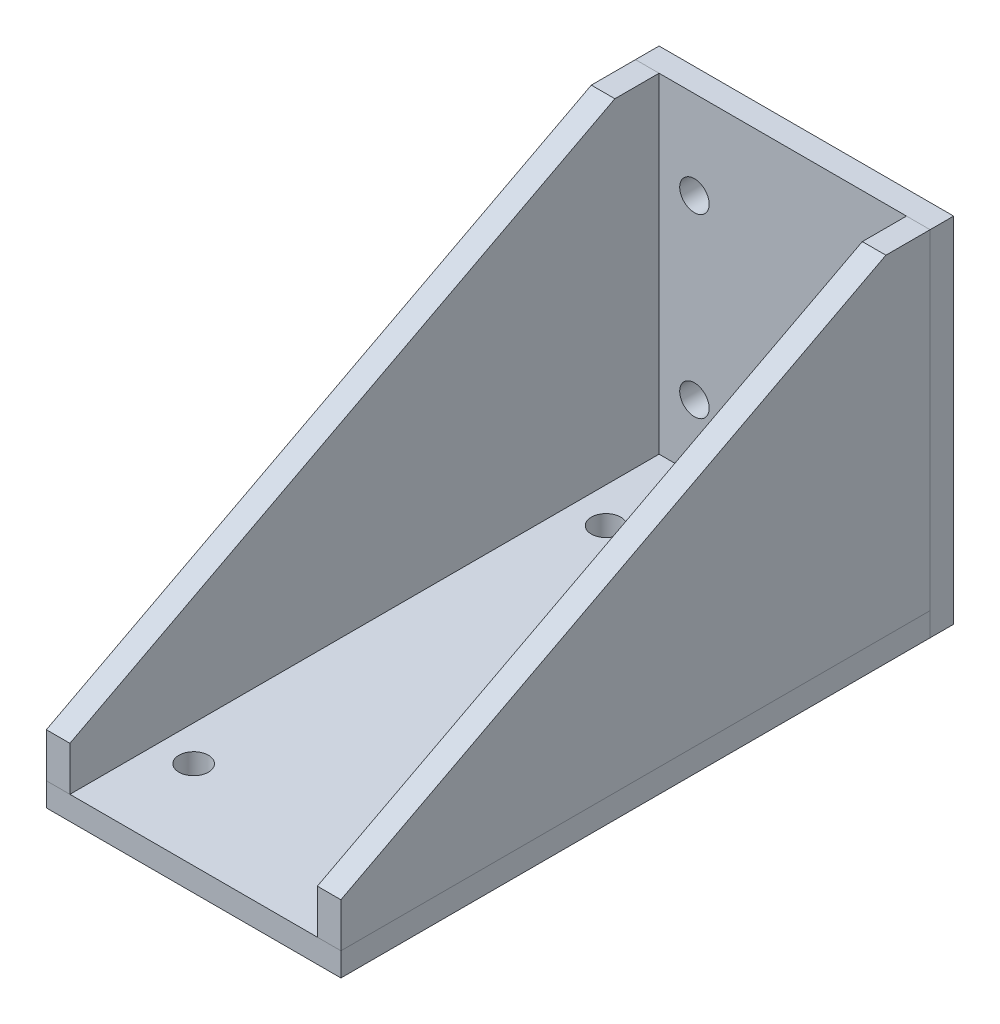
from build123d import *

# Parameters (mm, degrees)
SKETCH1_W                     = 100
SKETCH1_H                     = 120
BOSS_EXTRUDE1_DEPTH           = 8
SKETCH6_W                     = 100
SKETCH6_H                     = 8
BOSS_EXTRUDE4_DEPTH           = 200
BOSS_EXTRUDE2_DEPTH           = 8
BOSS_EXTRUDE3_DEPTH           = 8
M8_CLEARANCE_HOLE1_AT_2_COUNT = 2
M8_CLEARANCE_HOLE1_AT_2_PITCH = 60
M8_CLEARANCE_HOLE1_AT_3_COUNT = 2
M8_CLEARANCE_HOLE1_AT_3_PITCH = 140
M8_CLEARANCE_HOLE1_AT_4_COUNT = 2
M8_CLEARANCE_HOLE1_AT_4_PITCH = 152.315462117
M8_CLEARANCE_HOLE2_AT_2_COUNT = 2
M8_CLEARANCE_HOLE2_AT_2_PITCH = 60
M8_CLEARANCE_HOLE2_AT_3_COUNT = 2
M8_CLEARANCE_HOLE2_AT_3_PITCH = 84.852813742
M8_CLEARANCE_HOLE2_AT_4_COUNT = 2
M8_CLEARANCE_HOLE2_AT_4_PITCH = 60


with BuildPart() as part:
    # Sketch1 → Boss-Extrude1 (new body)
    with BuildSketch(Plane.XY):
        Rectangle(SKETCH1_W, SKETCH1_H)
    extrude(amount=BOSS_EXTRUDE1_DEPTH)

    # Sketch11 → M8 Clearance Hole2 (revolve, cut)
    with BuildSketch(Plane(origin=(30, 30, 0), x_dir=(0, 1, 0), z_dir=(1, 0, 0))):
        Polygon((0, 0), (0, 50.504303095), (5, 47.5), (5, 0), align=None)
    m8_clearance_hole2 = revolve(axis=Axis((30, 30, -6.35), (0, 0, 1)), mode=Mode.SUBTRACT)

    # M8 Clearance Hole2 at 2: M8 Clearance Hole2 ×2
    with Locations(*[(-i * M8_CLEARANCE_HOLE2_AT_2_PITCH, 0, 0) for i in range(1, M8_CLEARANCE_HOLE2_AT_2_COUNT)]):
        add(m8_clearance_hole2, mode=Mode.SUBTRACT)

    # M8 Clearance Hole2 at 3: M8 Clearance Hole2 ×2
    with Locations(*[Vector(-0.7071067811865478, -0.7071067811865474, 0) * (i * M8_CLEARANCE_HOLE2_AT_3_PITCH) for i in range(1, M8_CLEARANCE_HOLE2_AT_3_COUNT)]):
        add(m8_clearance_hole2, mode=Mode.SUBTRACT)

    # M8 Clearance Hole2 at 4: M8 Clearance Hole2 ×2
    with Locations(*[(0, -i * M8_CLEARANCE_HOLE2_AT_4_PITCH, 0) for i in range(1, M8_CLEARANCE_HOLE2_AT_4_COUNT)]):
        add(m8_clearance_hole2, mode=Mode.SUBTRACT)


with BuildPart() as body_2:
    # Sketch6 → Boss-Extrude4 (new body)
    with BuildSketch(Plane.XY.offset(8)):
        with Locations((0, -56)):
            Rectangle(SKETCH6_W, SKETCH6_H)
    extrude(amount=BOSS_EXTRUDE4_DEPTH)

    # Sketch8 → M8 Clearance Hole1 (revolve, cut)
    with BuildSketch(Plane(origin=(-30, -52, 38), x_dir=(0, 0, 1), z_dir=(1, 0, 0))):
        Polygon((0, 0), (0, 50.504303095), (5, 47.5), (5, 0), align=None)
    m8_clearance_hole1 = revolve(axis=Axis((-30, -45.65, 38), (0, -1, 0)), mode=Mode.SUBTRACT)

    # M8 Clearance Hole1 at 2: M8 Clearance Hole1 ×2
    with Locations(*[(i * M8_CLEARANCE_HOLE1_AT_2_PITCH, 0, 0) for i in range(1, M8_CLEARANCE_HOLE1_AT_2_COUNT)]):
        add(m8_clearance_hole1, mode=Mode.SUBTRACT)

    # M8 Clearance Hole1 at 3: M8 Clearance Hole1 ×2
    with Locations(*[(0, 0, i * M8_CLEARANCE_HOLE1_AT_3_PITCH) for i in range(1, M8_CLEARANCE_HOLE1_AT_3_COUNT)]):
        add(m8_clearance_hole1, mode=Mode.SUBTRACT)

    # M8 Clearance Hole1 at 4: M8 Clearance Hole1 ×2
    with Locations(*[Vector(0.39391929857916774, 0, 0.9191450300180579) * (i * M8_CLEARANCE_HOLE1_AT_4_PITCH) for i in range(1, M8_CLEARANCE_HOLE1_AT_4_COUNT)]):
        add(m8_clearance_hole1, mode=Mode.SUBTRACT)


with BuildPart() as body_3:
    # Sketch3 → Boss-Extrude2 (new body)
    with BuildSketch(Plane.ZY.offset(50)):
        Polygon((208, -52), (208, -37), (23, 60), (8, 60), (8, -52), align=None)
    extrude(amount=-BOSS_EXTRUDE2_DEPTH)


with BuildPart() as body_4:
    # Sketch4 → Boss-Extrude3 (new body)
    with BuildSketch(Plane(origin=(50, 0, 0), x_dir=(0, 0, -1), z_dir=(1, 0, 0))):
        Polygon((-8, -52), (-8, 60), (-23, 60), (-208, -37), (-208, -52), align=None)
    extrude(amount=-BOSS_EXTRUDE3_DEPTH)


solid = Compound([part.part, body_2.part, body_3.part, body_4.part])
